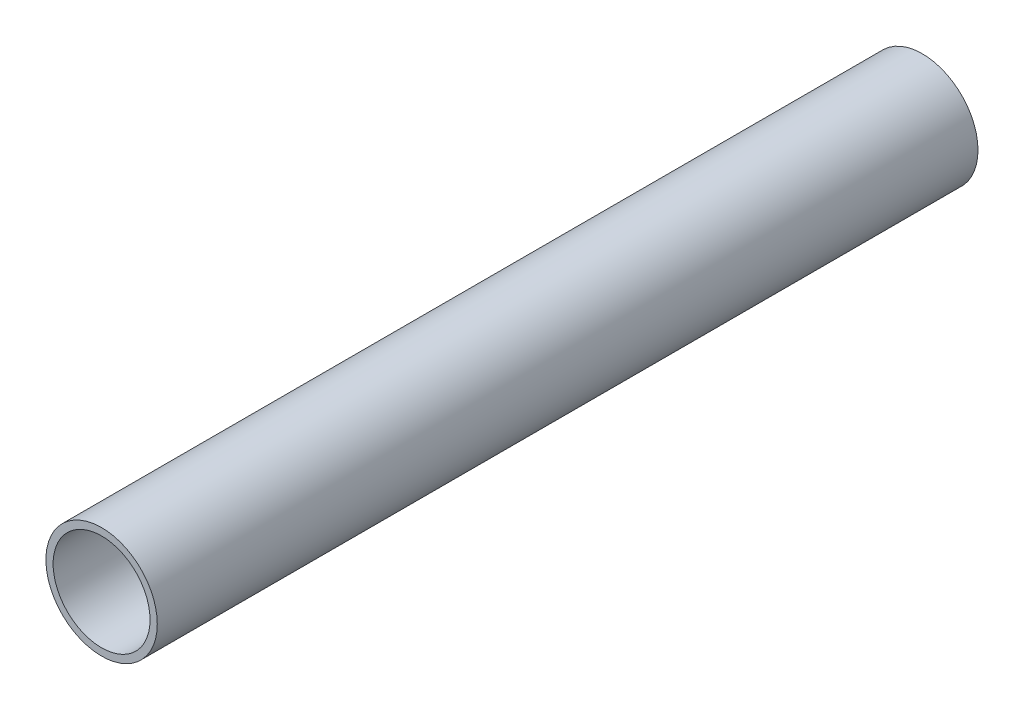
from build123d import *

# Parameters (mm, degrees)
BOSS_EXTRUDE1_DEPTH      = 222.25
BOSS_EXTRUDE1_DEPTH_BACK = 222.25
SKETCH1_R                = 30.1625
SKETCH1_R_2              = 26.2509


with BuildPart() as part:
    # Sketch1 → Boss-Extrude1 (new, two sides: drawn at the far end of the back side and taken through both)
    with BuildSketch(Plane.XY.offset(-BOSS_EXTRUDE1_DEPTH_BACK)):
        Circle(SKETCH1_R)
        Circle(SKETCH1_R_2, mode=Mode.SUBTRACT)
    extrude(amount=BOSS_EXTRUDE1_DEPTH + BOSS_EXTRUDE1_DEPTH_BACK)


solid = part.part
